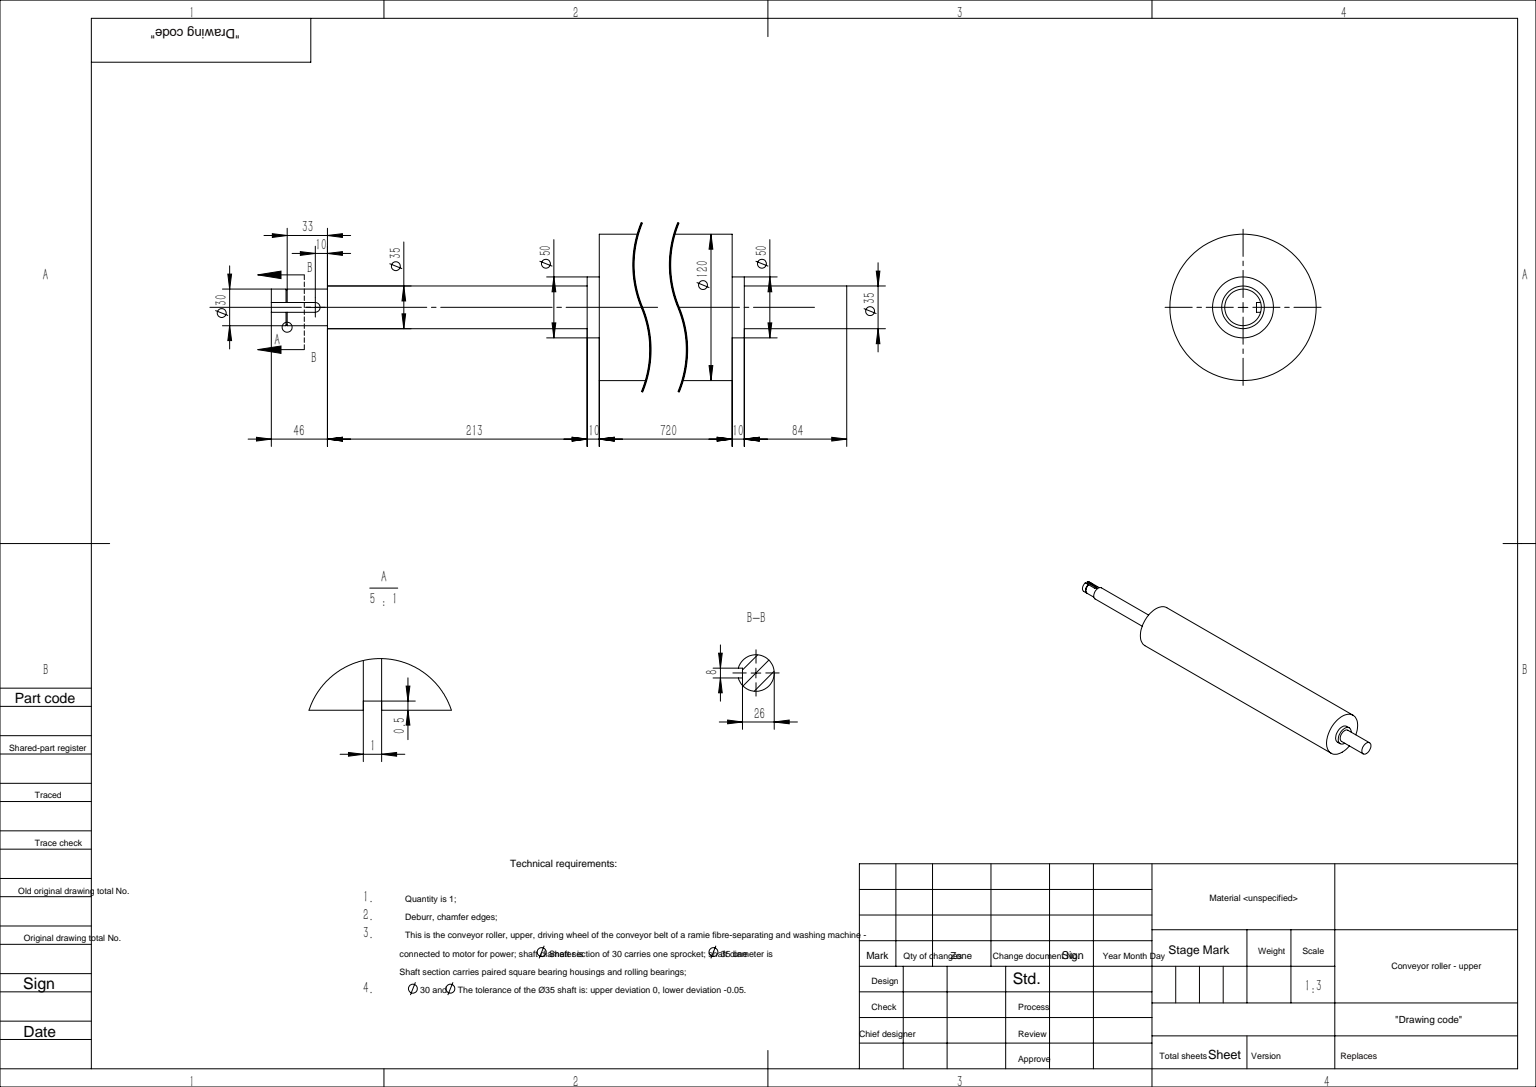
from build123d import *

# Parameters (mm, degrees)
CUT_EXTRUDE_1_DEPTH = 4
CUT_EXTRUDE_START   = 31.9
SKETCH_3_R          = 15
SKETCH_3_R_2        = 14.3
CUT_EXTRUDE_2_DEPTH = 1.3


with BuildPart() as part:
    # 草图1 → 旋转1 (revolve)
    with BuildSketch(Plane.XY, mode=Mode.PRIVATE) as revolve_1_sk:
        Polygon((-360, 60), (360, 60), (360, 25), (370, 25), (370, 17.5), (454, 17.5), (454, 0), (-629, 0), (-629, 15), (-583, 15), (-583, 17.5), (-370, 17.5), (-370, 25), (-360, 25), align=None)
    revolve(revolve_1_sk.sketch.rotate(Axis((-629, 0, 0), (1, 0, 0)), 180), axis=Axis((-629, 0, 0), (1, 0, 0)))

    # 草图2 → 切除-拉伸1 (cut)
    with BuildSketch(Plane(origin=(0, 15, 0), x_dir=(1, 0, 0), z_dir=(0, 1, 0))):
        with BuildLine():
            Line((-629, 4), (-593, 4))
            ThreePointArc((-593, 4), (-589, 0), (-593, -4))
            Line((-593, -4), (-629, -4))
            Line((-629, -4), (-629, 4))
        make_face()
    extrude(amount=-CUT_EXTRUDE_1_DEPTH, mode=Mode.SUBTRACT)

    # 草图3 → 切除-拉伸2 (cut)
    with BuildSketch(Plane.ZY.offset(583).offset(CUT_EXTRUDE_START)):
        with Locations(Location((0, 0, 0), (0, 0, 270))):
            Circle(SKETCH_3_R)
        Circle(SKETCH_3_R_2, mode=Mode.SUBTRACT)
    extrude(amount=CUT_EXTRUDE_2_DEPTH, mode=Mode.SUBTRACT)


solid = part.part
